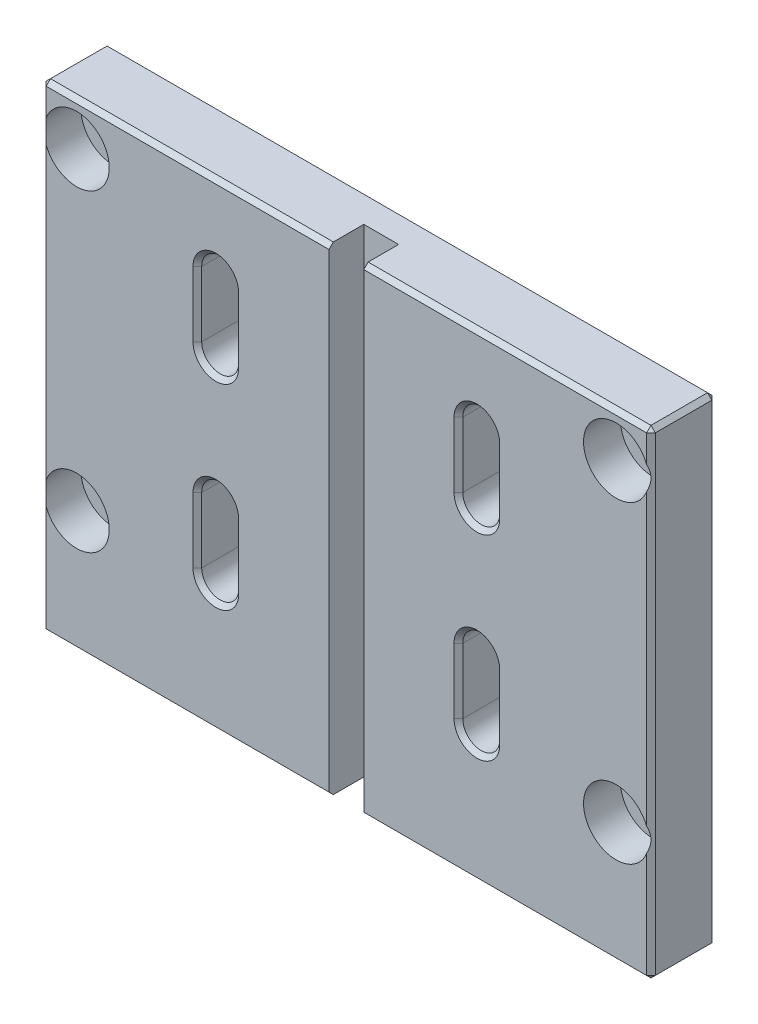
from build123d import *

# Parameters (mm, degrees)
SKETCH_1_W                   = 140
SKETCH_1_H                   = 110
EXTRUDE_1_DEPTH              = 7.5
CUT_EXTRUDE_1_DEPTH          = 91.277350426
CHAMFER_2_SIZE               = 1
SKETCH_5_W                   = 8
SKETCH_5_H                   = 16
CUT_EXTRUDE_2_DEPTH          = 131.599578866
HOLE_WIZARD_M5_1_D           = 4.2
HOLE_WIZARD_M5_2_D           = 4.2
HOLE_WIZARD_M5_2_DEPTH       = 12.4
HOLE_WIZARD_M5_2_CSINK_D     = 5.05
HOLE_WIZARD_M5_2_CSINK_ANGLE = 90
HOLE_WIZARD_M5_2_TIP         = 1.2618073
HOLE1_D                      = 9
HOLE1_CBORE_D                = 15
HOLE1_CBORE_DEPTH            = 8.5


with BuildPart() as part:
    # 草图1 → 凸台-拉伸1 (new, symmetric)
    with BuildSketch(Plane.XY):
        Rectangle(SKETCH_1_W, SKETCH_1_H)
    extrude(amount=EXTRUDE_1_DEPTH, both=True)

    # 草图4 → 切除-拉伸1 (cut, through all)
    with BuildSketch(Plane(origin=(0, 0, -7.5), x_dir=(-1, 0, 0), z_dir=(0, 0, -1))):
        with BuildLine():
            Line((-25.75, -10), (-25.75, -25))
            ThreePointArc((-25.75, -25), (-30, -29.25), (-34.25, -25))
            Line((-34.25, -25), (-34.25, -10))
            ThreePointArc((-34.25, -10), (-30, -5.75), (-25.75, -10))
        make_face()
        with BuildLine():
            Line((-25.75, 35), (-25.75, 20))
            ThreePointArc((-25.75, 20), (-30, 15.75), (-34.25, 20))
            Line((-34.25, 20), (-34.25, 35))
            ThreePointArc((-34.25, 35), (-30, 39.25), (-25.75, 35))
        make_face()
        with BuildLine():
            Line((25.75, 35), (25.75, 20))
            ThreePointArc((25.75, 20), (30, 15.75), (34.25, 20))
            Line((34.25, 20), (34.25, 35))
            ThreePointArc((34.25, 35), (30, 39.25), (25.75, 35))
        make_face()
        with BuildLine():
            Line((25.75, -10), (25.75, -25))
            ThreePointArc((25.75, -25), (30, -29.25), (34.25, -25))
            Line((34.25, -25), (34.25, -10))
            ThreePointArc((34.25, -10), (30, -5.75), (25.75, -10))
        make_face()
    extrude(amount=-CUT_EXTRUDE_1_DEPTH, mode=Mode.SUBTRACT)

    # 倒角2
    chamfer_2_edges = [part.edges().sort_by_distance(p)[0] for p in [
        (70, 0, 7.5),
        (0, 55, 7.5),
        (30, -5.75, 7.5),
        (25.75, -17.5, 7.5),
        (30, -29.25, 7.5),
        (34.25, -17.5, 7.5),
        (30, -5.75, -7.5),
        (34.25, -17.5, -7.5),
        (30, -29.25, -7.5),
        (25.75, -17.5, -7.5),
        (30, 39.25, 7.5),
        (25.75, 27.5, 7.5),
        (-70, 0, 7.5),
        (30, 15.75, 7.5),
        (34.25, 27.5, 7.5),
        (30, 39.25, -7.5),
        (34.25, 27.5, -7.5),
        (30, 15.75, -7.5),
        (25.75, 27.5, -7.5),
        (0, 55, -7.5),
        (-30, 39.25, 7.5),
        (-34.25, 27.5, 7.5),
        (-30, 15.75, 7.5),
        (-25.75, 27.5, 7.5),
        (-30, 39.25, -7.5),
        (-25.75, 27.5, -7.5),
        (-30, 15.75, -7.5),
        (-34.25, 27.5, -7.5),
        (70, 0, -7.5),
        (-30, -5.75, 7.5),
        (-34.25, -17.5, 7.5),
        (-30, -29.25, 7.5),
        (-25.75, -17.5, 7.5),
        (-30, -5.75, -7.5),
        (-25.75, -17.5, -7.5),
        (0, -55, -7.5),
        (-30, -29.25, -7.5),
        (-34.25, -17.5, -7.5),
        (-70, 0, -7.5),
        (0, -55, 7.5),
        (-70, 55, 0),
        (70, 55, 0),
        (70, -55, 0),
        (-70, -55, 0),
    ]]
    chamfer(chamfer_2_edges, length=CHAMFER_2_SIZE)

    # 草图5 → 切除-拉伸2 (cut, through all)
    with BuildSketch(Plane(origin=(0, 55, 0), x_dir=(1, 0, 0), z_dir=(0, 1, 0))):
        with Locations((0, -7.5)):
            Rectangle(SKETCH_5_W, SKETCH_5_H)
    extrude(amount=-CUT_EXTRUDE_2_DEPTH, mode=Mode.SUBTRACT)

    # M5 螺纹孔1 (through all)
    with Locations(Plane(origin=(0, 0, -7.5), x_dir=(-1, 0, 0), z_dir=(0, 0, -1))):
        with Locations((-62, 45), (-62, -27), (62, -27), (62, 45)):
            Hole(HOLE_WIZARD_M5_1_D / 2)

    # M5 螺纹孔2
    with Locations(Plane(origin=(0, -55, 0), x_dir=(-1, 0, 0), z_dir=(0, -1, 0))):
        with Locations((45, 0), (-45, 0)):
            CounterSinkHole(HOLE_WIZARD_M5_2_D / 2, HOLE_WIZARD_M5_2_CSINK_D / 2, depth=HOLE_WIZARD_M5_2_DEPTH, counter_sink_angle=HOLE_WIZARD_M5_2_CSINK_ANGLE)
            with Locations((0, 0, -(HOLE_WIZARD_M5_2_DEPTH + HOLE_WIZARD_M5_2_TIP / 2))):  # 118° drill point
                Cone(0, HOLE_WIZARD_M5_2_D / 2, HOLE_WIZARD_M5_2_TIP, mode=Mode.SUBTRACT)

    # Hole1 (through all)
    with Locations(Plane(origin=(49.130892878, -26.065000019, 7.5), x_dir=(1, 0, 0), z_dir=(0, 0, 1))):
        with Locations((12.869107122, -0.934999981), (12.869107122, 71.065000019), (-111.130892878, 71.065000019), (-111.130892878, -0.934999981)):
            CounterBoreHole(HOLE1_D / 2, HOLE1_CBORE_D / 2, HOLE1_CBORE_DEPTH)


solid = part.part
